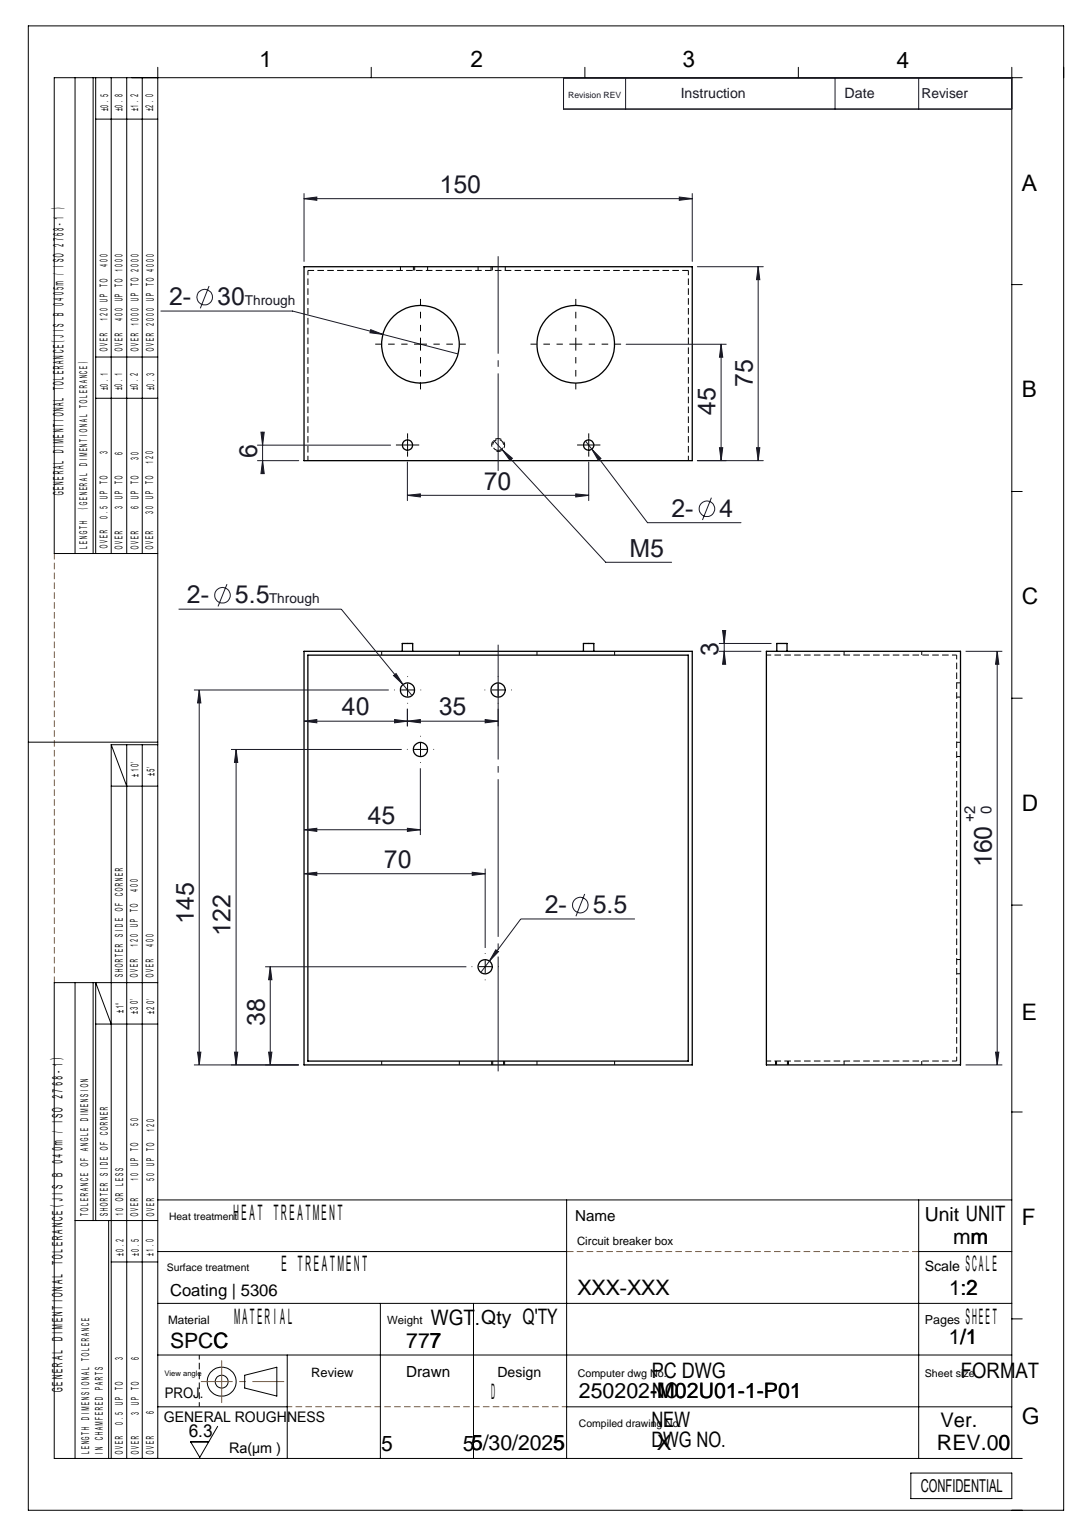
SolidWorks part; units mm, degrees
material "SPCC"
ref_plane "Front Plane" through (0, 0, 0) normal (0, 0, 1) x (1, 0, 0)
ref_plane "Top Plane" through (0, 0, 0) normal (0, 1, 0) x (1, 0, 0)
ref_plane "Right Plane" through (0, 0, 0) normal (1, 0, 0) x (0, 0, -1)
sketch "Sketch1" plane through (0, 0, 0) normal (0, 0, 1) x (1, 0, 0)
  line L1 (-75, 80) -> (75, 80)
  line L2 (-75, 80) -> (-75, -80)
  line L3 (-75, -80) -> (75, -80)
  line L4 (75, 80) -> (75, -80)
  line L5 (-75, 80) -> (75, -80) construction
  line L6 (-75, -80) -> (75, 80) construction
  point P0 (0, 0)
  dimension "D1" = 150
  dimension "D2" = 160
extrude "Boss-Extrude1" add sketch "Sketch1" along normal mid plane 75
shell "Shell1" thickness 1.5
hole_wizard "Ø5.5 (5.5) Diameter Hole2" positions "Sketch4" profile "Sketch3" hole size "Ø5.5" standard "GB" end condition through all
sketch "Sketch4" plane through (0, 0, -36) normal (0, 0, 1) x (1, 0, 0)
  point P0 (-30, 42)
  point P2 (-5, -42)
  dimension "D1" = 84
  dimension "D2" = 42
  dimension "D3" = 25
  dimension "D4" = 30
sketch "Sketch3" plane through (-30, 42, -36) normal (1, 0, 0) x (0, -1, 0)
  line L0 (0, 0) -> (0, 1.5)
  line L1 (0, 1.5) -> (2.75, 1.5)
  line L2 (2.75, 1.5) -> (2.75, 0)
  line L5 (2.75, 0) -> (0, 0)
  line L11 (0, -6.35) -> (0, 107.95) construction
  dimension "通孔孔直径" = 5.5
  dimension "通孔孔深度" = 1.5
sketch "Sketch6" plane through (0, 80, 0) normal (0, 1, 0) x (1, 0, 0)
  line L0 (0, -2.5237) -> (0, 63.5106) construction
  line L1 (75, 37.5) -> (-75, 37.5) construction
  circle A0 centre (-30, 7.5) radius 15
  circle A1 centre (30, 7.5) radius 15
  dimension "D2" = 30
  dimension "D1" = 30
  dimension "D3" = 60
extrude "Cut-Extrude2" cut sketch "Sketch6" against normal through all
sketch "Sketch8" plane through (0, 80, 0) normal (0, 1, 0) x (1, 0, 0)
  line L0 (0, 0) -> (0, -48.0785) construction
  line L1 (75, -37.5) -> (-75, -37.5) construction
  line L3 (-40, -30.5) -> (-30, -30.5) construction
  line L4 (-40, -30.5) -> (-40, -32.5) construction
  line L5 (-40, -32.5) -> (-30, -32.5) construction
  line L6 (-30, -30.5) -> (-30, -32.5) construction
  line L7 (-40, -30.5) -> (-30, -32.5) construction
  line L8 (-40, -32.5) -> (-30, -30.5) construction
  line L9 (30, -30.5) -> (40, -30.5) construction
  line L10 (30, -30.5) -> (30, -32.5) construction
  line L11 (30, -32.5) -> (40, -32.5) construction
  line L12 (40, -30.5) -> (40, -32.5) construction
  line L13 (30, -30.5) -> (40, -32.5) construction
  line L14 (30, -32.5) -> (40, -30.5) construction
  circle A0 centre (-35, -31.5) radius 2
  circle A1 centre (35, -31.5) radius 2
  point P0 (-35, -31.5)
  point P5 (35, -31.5)
  dimension "D3" = 35
  dimension "D9" = 4
  dimension "D10" = 4
  dimension "D1" = 10
  dimension "D2" = 10
  dimension "D4" = 2
  dimension "D5" = 6
  dimension "D6" = 35
  dimension "D7" = 6
  dimension "D8" = 2
extrude "Boss-Extrude2" add sketch "Sketch8" along normal blind 3
hole_wizard "M5 Tapped Hole1" positions "Sketch10" profile "Sketch9" tap size "M5" standard "GB"
sketch "Sketch10" plane through (0, -80, 0) normal (0, -1, 0) x (1, 0, 0)
  line L0 (-75, 37.5) -> (75, 37.5) construction
  line L1 (0, 0) -> (0, 50.2443) construction
  point P0 (0, 31.5)
  dimension "D1" = 6
sketch "Sketch9" plane through (0, -80, 31.5) normal (1, 0, 0) x (0, 0, -1)
  line L0 (0, 0) -> (0, 15.2618)
  line L1 (0, 15.2618) -> (2.1, 14)
  line L2 (2.1, 14) -> (2.1, 0)
  line L5 (2.1, 0) -> (0, 0)
  line L10 (0, 15.2618) -> (-2.1, 14) construction
  line L11 (0, -6.35) -> (0, 107.95) construction
  dimension "螺纹孔钻头直径" = 4.2
  dimension "螺纹孔钻头深度" = 14
  dimension "导头角度" = 118
cosmetic thread "Cosmetic Thread1" parameters "D1"=1.5, "D2"=5
hole_wizard "Ø5.5 (5.5) Diameter Hole1" positions "Sketch12" profile "Sketch11" hole size "Ø5.5" standard "GB"
sketch "Sketch12" plane through (0, 0, -36) normal (0, 0, 1) x (1, 0, 0)
  line L1 (0, 0) -> (51.4583, 0) construction
  point P0 (0, 65)
  point P15 (-35, 65)
  dimension "D1" = 35
  dimension "D2" = 65
sketch "Sketch11" plane through (0, 65, -36) normal (1, 0, 0) x (0, -1, 0)
  line L0 (0, 0) -> (0, 16.6524)
  line L1 (0, 16.6524) -> (2.75, 15)
  line L2 (2.75, 15) -> (2.75, 0)
  line L5 (2.75, 0) -> (0, 0)
  line L10 (0, 16.6524) -> (-2.75, 15) construction
  line L11 (0, -6.35) -> (0, 107.95) construction
  dimension "孔直径" = 5.5
  dimension "孔深度" = 15
  dimension "导头角度" = 118
